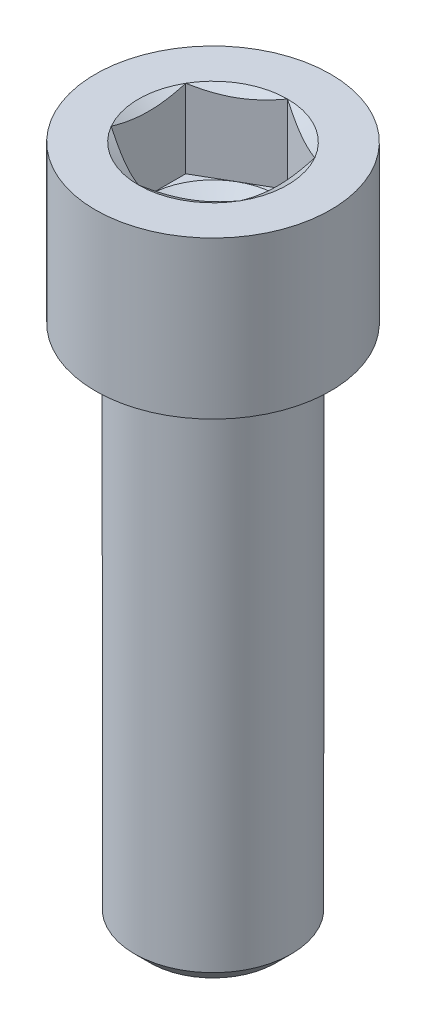
SolidWorks part; units mm, degrees
material "45"
ref_plane "Front Plane" through (0, 0, 0) normal (0, 0, 1) x (1, 0, 0)
ref_plane "Top Plane" through (0, 0, 0) normal (0, 1, 0) x (1, 0, 0)
ref_plane "Right Plane" through (0, 0, 0) normal (1, 0, 0) x (0, 0, -1)
sketch "Sketch1" plane through (0, 0, 0) normal (0, 1, 0) x (1, 0, 0)
  circle A0 centre (0, 0) radius 9
  dimension "D1" = 18
extrude "Boss-Extrude1" add sketch "Sketch1" along normal blind 12
sketch "Sketch2" plane through (0, 0, 0) normal (0, -1, 0) x (1, 0, 0)
  circle A0 centre (0, 0) radius 6
  dimension "D1" = 12
extrude "Boss-Extrude2" add sketch "Sketch2" along normal blind 40
cosmetic thread "Cosmetic Thread1" parameters "D1"=34.8, "D2"=10.106
sketch "Sketch3" plane through (0, 12, 0) normal (0, 1, 0) x (1, 0, 0)
  line L1 (0, 5.7) -> (-4.9363, 2.85)
  line L2 (-4.9363, 2.85) -> (-4.9363, -2.85)
  line L3 (-4.9363, -2.85) -> (0, -5.7)
  line L4 (0, -5.7) -> (4.9363, -2.85)
  line L5 (4.9363, -2.85) -> (4.9363, 2.85)
  line L6 (4.9363, 2.85) -> (0, 5.7)
  circle A0 centre (0, 0) radius 5.7 construction
  dimension "D1" = 11.4
extrude "Cut-Extrude1" cut sketch "Sketch3" against normal blind 6
sketch "Sketch4" plane through (0, 0, 0) normal (0, 0, 1) x (1, 0, 0)
  line L0 (0, 6) -> (4.9363, 6) construction
  line L1 (4.9363, 6) -> (4.9363, 12) construction
  line L2 (9, 12) -> (-9, 12) construction
  line L3 (0, 6) -> (4.9363, 6)
  line L4 (4.9363, 11.5591) -> (4.9363, 12)
  line L5 (5.7, 12) -> (4.9363, 12)
  line L6 (0, -3.9322) -> (0, 16.6801) construction
  line L7 (4.9363, 6) -> (0, 3.15)
  line L8 (0, 3.15) -> (0, 6)
  line L9 (5.7, 12) -> (4.9363, 11.5591)
  dimension "D1" = 60
  dimension "D2" = 11.4
  dimension "D3" = 60
revolve "Cut-Revolve1" cut sketch "Sketch4" angle 360 about L6
chamfer "Chamfer1" distance 1.2 angle 45 1 edges at (0, -40, -6)
